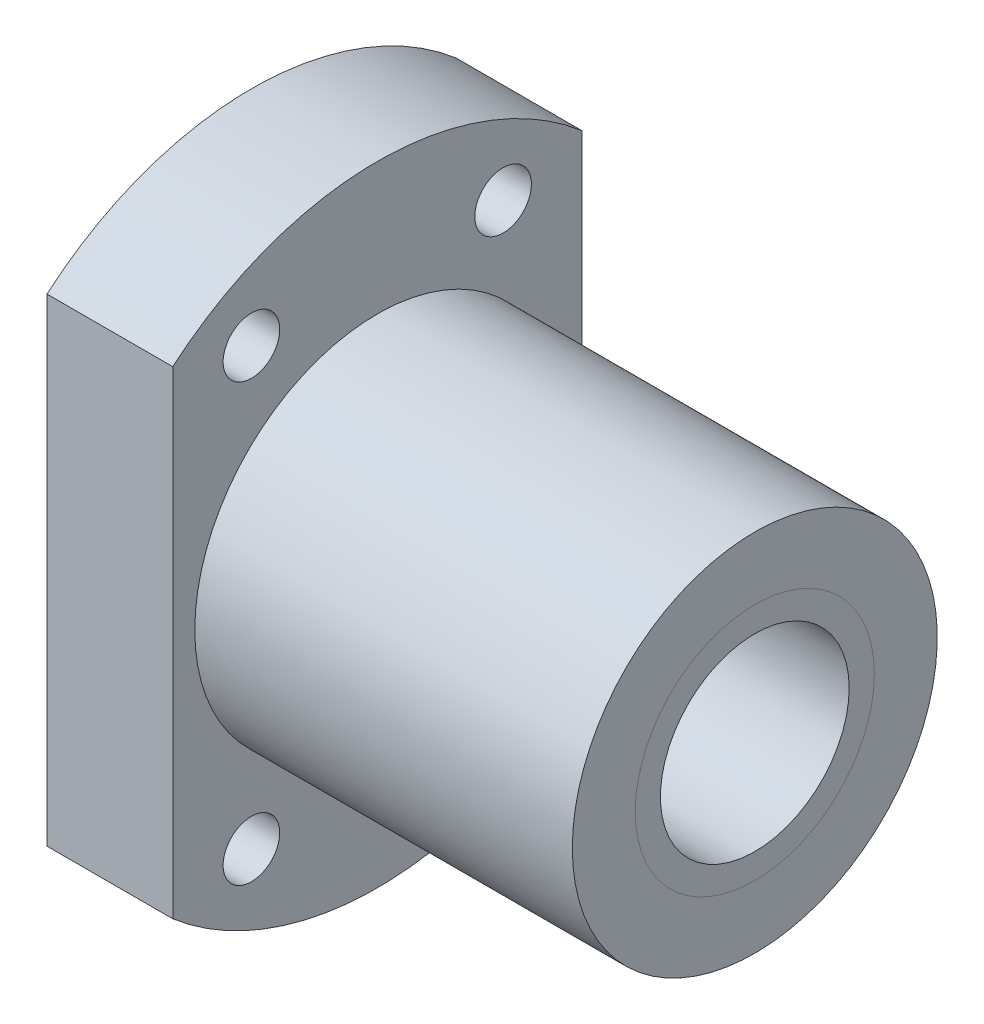
SolidWorks part; units mm, degrees
ref_plane "Front Plane" through (0, 0, 0) normal (0, 0, 1) x (1, 0, 0)
ref_plane "Top Plane" through (0, 0, 0) normal (0, 1, 0) x (1, 0, 0)
ref_plane "Right Plane" through (0, 0, 0) normal (1, 0, 0) x (0, 0, -1)
sketch "Sketch1" plane through (0, 0, 0) normal (0, 0, 1) x (1, 0, 0)
  line L0 (0, 0) -> (101.3644, 0) construction
  line L1 (0, 19) -> (0, 50)
  line L2 (0, 50) -> (20, 50)
  line L3 (20, 50) -> (20, 29)
  line L4 (20, 29) -> (80, 29)
  line L5 (80, 29) -> (80, 19)
  line L6 (80, 19) -> (0, 19)
  dimension "D1" = 38
  dimension "D2" = 10
  dimension "D3" = 100
  dimension "D4" = 20
  dimension "D5" = 80
revolve "Revolve1" add sketch "Sketch1" angle 360 about L0
hole_wizard "Hole size per socket head cap screw type1" positions "Sketch3" profile "Sketch2" counterbore size "M8" standard "GB" end condition through all
sketch "Sketch3" plane through (0, 0, 0) normal (-1, 0, 0) x (0, 0, 1)
  line L0 (0, 40) -> (0, 0) construction
  line L2 (-20, 34.641) -> (0, 0) construction
  circle A0 centre (0, 0) radius 40 construction
  point P0 (20, 34.641)
  point P1 (-20, 34.641)
  point P5 (-20, -34.641)
  point P7 (20, -34.641)
  dimension "D1" = 80
  dimension "D2" = 30
sketch "Sketch2" plane through (0, 34.641, 20) normal (0, 1, 0) x (0, 0, 1)
  line L0 (0, 0) -> (0, 80)
  line L1 (0, 80) -> (4.5, 80)
  line L3 (4.5, 80) -> (4.5, 9)
  line L4 (4.5, 9) -> (7.5, 9)
  line L5 (7.5, 9) -> (7.5, 0)
  line L7 (7.5, 0) -> (0, 0)
  line L11 (0, -6.35) -> (0, 107.95) construction
  dimension "通孔孔直径" = 9
  dimension "通孔孔深度" = 80
  dimension "柱形沉头孔直径" = 15
  dimension "柱形沉头孔深度" = 9
sketch "Sketch4" plane through (0, 0, 0) normal (-1, 0, 0) x (0, 0, 1)
  line L1 (-32.5, -55) -> (32.5, -55)
  line L2 (-32.5, -55) -> (-32.5, 55)
  line L3 (-32.5, 55) -> (32.5, 55)
  line L4 (32.5, -55) -> (32.5, 55)
  line L5 (-32.5, -55) -> (32.5, 55) construction
  line L6 (-32.5, 55) -> (32.5, -55) construction
  point P0 (0, 0)
  dimension "D1" = 110
  dimension "D2" = 65
extrude "Cut-Extrude1" cut sketch "Sketch4" against normal through all flip side to cut
sketch "Sketch5" plane through (80, 0, 0) normal (1, 0, 0) x (0, 0, -1)
  circle A0 centre (0, 0) radius 19
  circle A1 centre (0, 0) radius 15
  dimension "D1" = 38
  dimension "D2" = 30
extrude "Boss-Extrude1" add sketch "Sketch5" against normal blind 40 separate body
sketch "Sketch6" plane through (0, 0, 0) normal (-1, 0, 0) x (0, 0, 1)
  circle A0 centre (0, 0) radius 19
  circle A1 centre (0, 0) radius 15
  dimension "D1" = 38
  dimension "D2" = 30
extrude "Boss-Extrude2" add sketch "Sketch6" against normal blind 40 separate body
